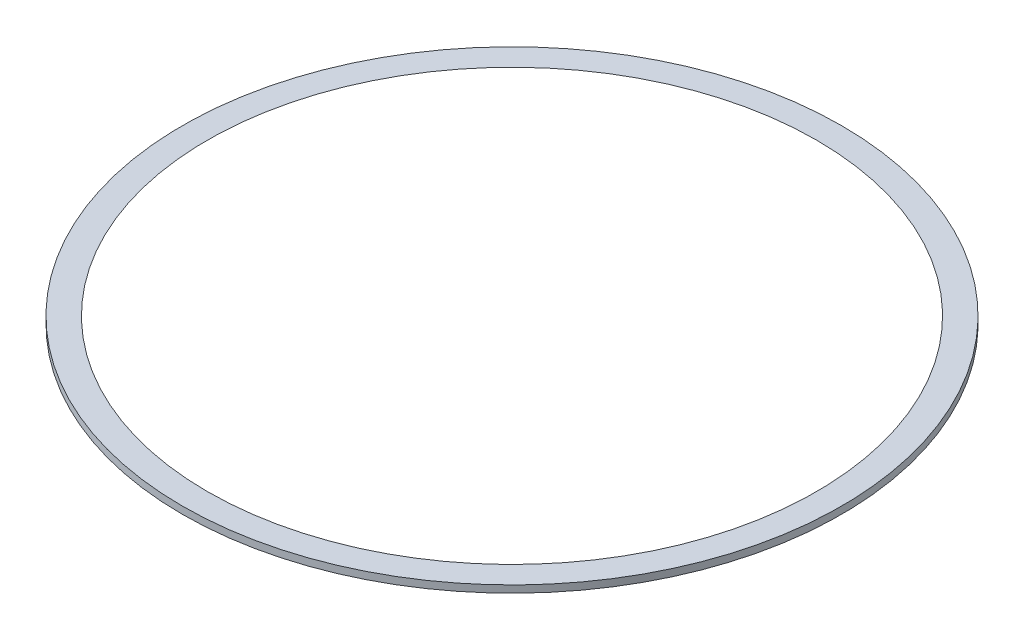
SolidWorks part; units mm, degrees
ref_plane "Front Plane" through (0, 0, 0) normal (0, 0, 1) x (1, 0, 0)
ref_plane "Top Plane" through (0, 0, 0) normal (0, 1, 0) x (1, 0, 0)
ref_plane "Right Plane" through (0, 0, 0) normal (1, 0, 0) x (0, 0, -1)
sketch "Sketch1" plane through (0, 0, 0) normal (0, 0, 1) x (1, 0, 0)
  line L0 (-170, 4) -> (-184, 4)
  line L1 (-184, 4) -> (-184, 0)
  line L2 (55, 0) -> (-55, 0) construction
  line L3 (-184, 0) -> (-176, 0)
  line L4 (-176, 0) -> (-170, 4)
  line L6 (0, -55) -> (0, 55) construction
  line L7 (0, 23.7582) -> (0, 50023.7582) construction
  dimension "D1" = 4
  dimension "D2" = 8
  dimension "D3" = 14
  dimension "D4" = 176
revolve "Revolve1" add sketch "Sketch1" angle 360 about L7
